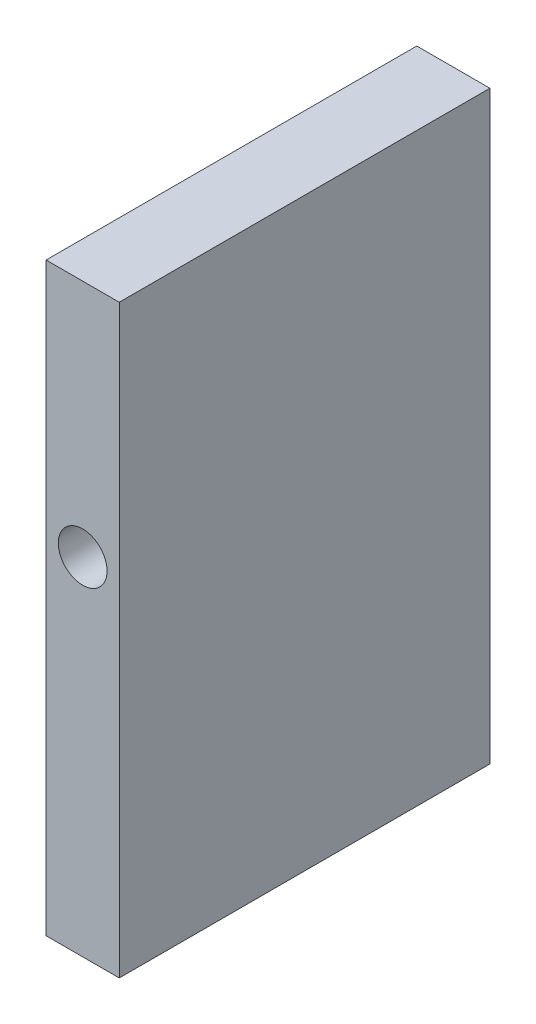
from build123d import *

# Parameters (mm, degrees)
SKETCH1_W           = 15
SKETCH1_H           = 120
BOSS_EXTRUDE1_DEPTH = 76
SKETCH2_R           = 5
CUT_EXTRUDE2_DEPTH  = 98.119771417


with BuildPart() as part:
    # Sketch1 → Boss-Extrude1 (new body)
    with BuildSketch(Plane.XY):
        Rectangle(SKETCH1_W, SKETCH1_H)
    extrude(amount=BOSS_EXTRUDE1_DEPTH)

    # Sketch2 → Cut-Extrude2 (cut, through all)
    with BuildSketch(Plane.XY.offset(76)):
        with Locations((0, 11)):
            Circle(SKETCH2_R)
    extrude(amount=-CUT_EXTRUDE2_DEPTH, mode=Mode.SUBTRACT)


solid = part.part
